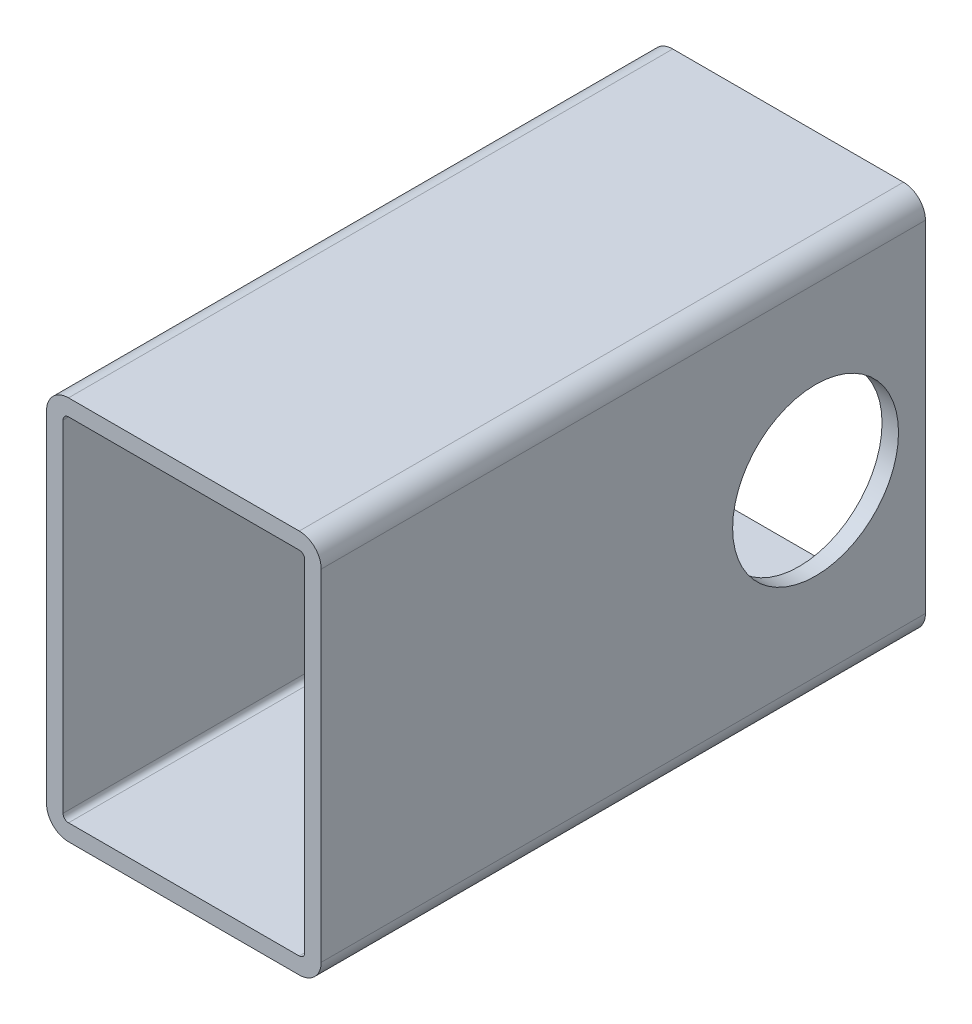
from build123d import *

# Parameters (mm, degrees)
EXTRUDE_THIN1_DEPTH = 110
SKETCH2_R           = 15.1
CUT_EXTRUDE1_DEPTH  = 126.797456254


with BuildPart() as part:
    # Sketch1 → Extrude-Thin1 (new body)
    with BuildSketch(Plane.XY):
        with BuildLine():
            Line((-25, 31), (-25, -31))
            ThreePointArc((-25, -31), (-23.828427125, -33.828427125), (-21, -35))
            Line((-21, -35), (21, -35))
            ThreePointArc((21, -35), (23.828427125, -33.828427125), (25, -31))
            Line((25, -31), (25, 31))
            ThreePointArc((25, 31), (23.828427125, 33.828427125), (21, 35))
            Line((21, 35), (-21, 35))
            ThreePointArc((-21, 35), (-23.828427125, 33.828427125), (-25, 31))
        make_face()
        with BuildLine():
            Line((-22, 31), (-22, -31))
            ThreePointArc((-22, -31), (-21.707106781, -31.707106781), (-21, -32))
            Line((-21, -32), (21, -32))
            ThreePointArc((21, -32), (21.707106781, -31.707106781), (22, -31))
            Line((22, -31), (22, 31))
            ThreePointArc((22, 31), (21.707106781, 31.707106781), (21, 32))
            Line((21, 32), (-21, 32))
            ThreePointArc((-21, 32), (-21.707106781, 31.707106781), (-22, 31))
        make_face(mode=Mode.SUBTRACT)
    extrude(amount=EXTRUDE_THIN1_DEPTH)

    # Sketch2 → Cut-Extrude1 (cut, through all)
    with BuildSketch(Plane(origin=(25, 0, 0), x_dir=(0, 0, -1), z_dir=(1, 0, 0))):
        with Locations((-20, 0)):
            Circle(SKETCH2_R)
    extrude(amount=-CUT_EXTRUDE1_DEPTH, mode=Mode.SUBTRACT)


solid = part.part
